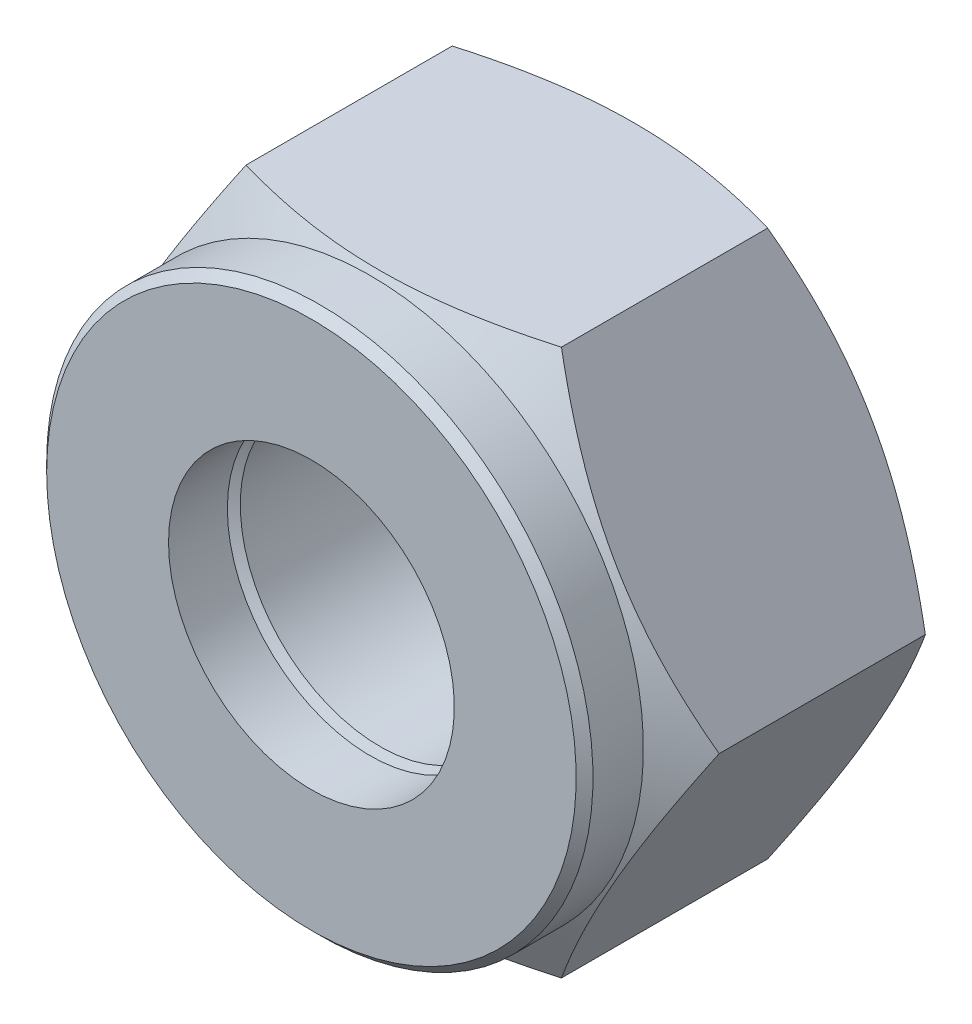
from build123d import *
from OCP.BRepFilletAPI import BRepFilletAPI_MakeChamfer

# Parameters (mm, degrees)
SKETCH1_R        = 3.3235
BASENUT_DEPTH    = 6.5
ENDCHAMFER_SIZE  = 0.4
ENDCHAMFER_SIZE2 = 0.230940108
SKETCH_1_R       = 6.5
SKETCH_1_R_2     = 3.4
EXTRUDE_1_DEPTH  = 1.4
CHAMFER_1_SIZE   = 0.2


with BuildPart() as part:
    # Sketch1 → BaseNut (new body)
    with BuildSketch(Plane.XY):
        Polygon((3.75277675, -6.5), (7.505553499, 0), (3.75277675, 6.5), (-3.75277675, 6.5), (-7.505553499, 0), (-3.75277675, -6.5), align=None)
        Circle(SKETCH1_R, mode=Mode.SUBTRACT)
    extrude(amount=-BASENUT_DEPTH)

    # Sketch2 → Double-Chamfer (revolve, cut)
    with BuildSketch(Plane(origin=(0, 0, 0), x_dir=(1, 0, 0), z_dir=(0, 1, 0))):
        Polygon((-7.505553499, 6.5), (-6.125, 6.5), (-7.505553499, 5.702937065), align=None)
        Polygon((-7.505553499, 0.797062935), (-7.505553499, 0), (-6.125, 0), align=None)
    revolve(axis=Axis((0, 0, -3.375940562), (0, 0, 1)), mode=Mode.SUBTRACT)

    # EndChamfer: one chamfer whose edges measure the first distance from different faces: ONE call of the kernel's chamfer builder (chamfer() names one face for all edges)
    endchamfer_edges_1 = [part.edges().sort_by_distance(p)[0] for p in [
        (-3.3235, 0, -6.5),
    ]]
    endchamfer_side_1 = [part.faces().sort_by_distance(p)[0] for p in [
        (-3.3235, 0, -3.25),
    ]]
    endchamfer_edges_2 = [part.edges().sort_by_distance(p)[0] for p in [
        (-3.3235, 0, 0),
    ]]
    endchamfer_side_2 = [part.faces().sort_by_distance(p)[0] for p in [
        (5.951758839, 0, 0),
    ]]
    endchamfer = BRepFilletAPI_MakeChamfer(part.part.solid().wrapped)
    for e in endchamfer_edges_1:
        endchamfer.Add(ENDCHAMFER_SIZE, ENDCHAMFER_SIZE2, e.wrapped, endchamfer_side_1[0].wrapped)  # the first distance lies on this face
    for e in endchamfer_edges_2:
        endchamfer.Add(ENDCHAMFER_SIZE, ENDCHAMFER_SIZE2, e.wrapped, endchamfer_side_2[0].wrapped)  # the first distance lies on this face
    add(Compound.cast(endchamfer.Shape()), mode=Mode.REPLACE)

    # 草图1 → 凸台-拉伸1 (add)
    with BuildSketch(Plane.XY):
        Circle(SKETCH_1_R)
        Circle(SKETCH_1_R_2, mode=Mode.SUBTRACT)
    extrude(amount=EXTRUDE_1_DEPTH)

    # 倒角1
    chamfer_1_edges = [part.edges().sort_by_distance(p)[0] for p in [
        (-6.5, 0, 1.4),
    ]]
    chamfer(chamfer_1_edges, length=CHAMFER_1_SIZE)


solid = part.part
